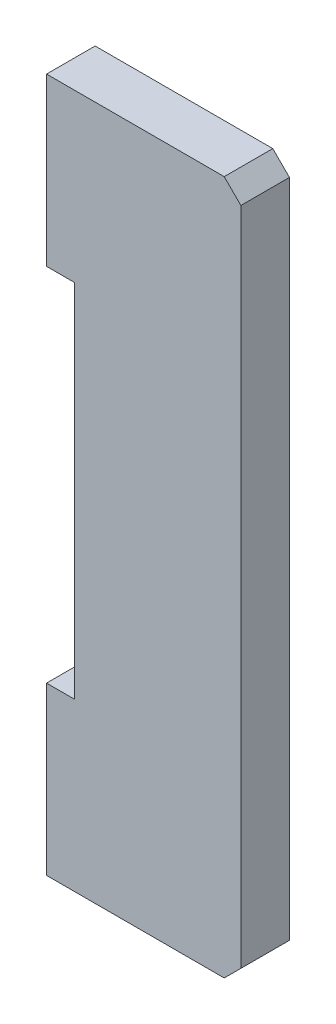
from build123d import *

# Parameters (mm, degrees)
EXTRUDE_1_DEPTH = 35
CHAMFER_1_SIZE  = 12


with BuildPart() as part:
    # 草图1 → 凸台-拉伸1 (new body)
    with BuildSketch(Plane.XY):
        Polygon((-140, 0), (0, 0), (0, -500), (-140, -500), (-140, -380), (-120, -380), (-120, -120), (-140, -120), align=None)
    extrude(amount=EXTRUDE_1_DEPTH)

    # 倒角1
    chamfer_1_edges = [part.edges().sort_by_distance(p)[0] for p in [
        (0, -500, 17.5),
        (0, 0, 17.5),
    ]]
    chamfer(chamfer_1_edges, length=CHAMFER_1_SIZE)


solid = part.part
